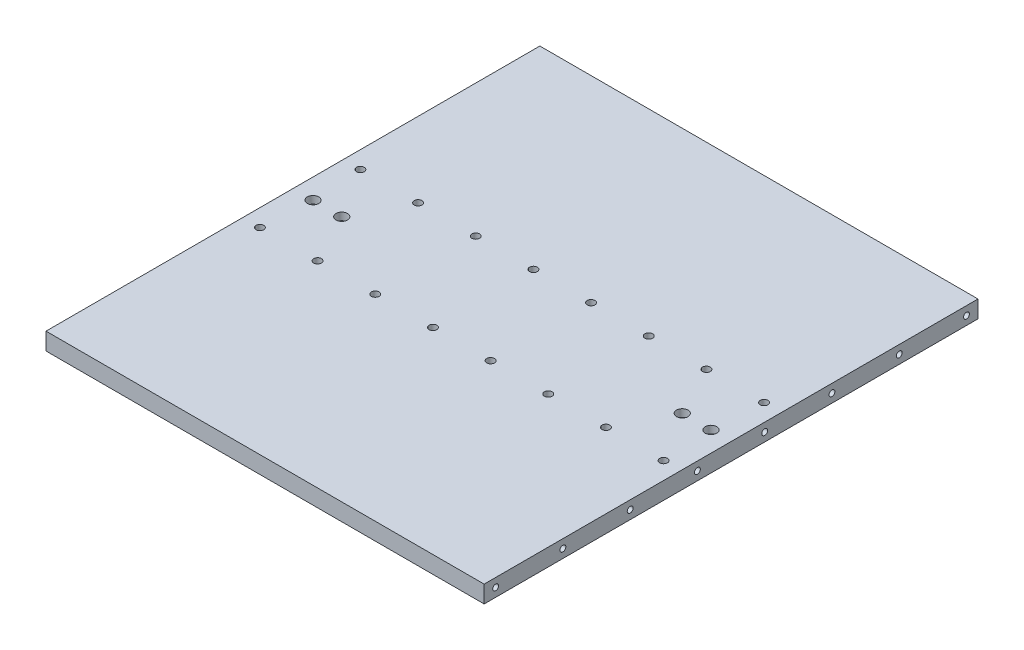
from build123d import *

# Parameters (mm, degrees)
SKETCH_1_W                = 763
SKETCH_1_H                = 860
EXTRUDE_1_DEPTH           = 30
HOLE_WIZARD_1_D           = 13.5
HOLE_WIZARD_1_CBORE_D     = 20
HOLE_WIZARD_1_CBORE_DEPTH = 13
HOLE_WIZARD_2_D           = 13.5
HOLE_WIZARD_2_CBORE_D     = 20
HOLE_WIZARD_2_CBORE_DEPTH = 13
HOLE_WIZARD_M12_1_D       = 10.2
HOLE_WIZARD_M12_1_DEPTH   = 29.25
HOLE_WIZARD_M12_1_TIP     = 3.064389157
HOLE_WIZARD_M12_2_D       = 10.2
HOLE_WIZARD_M12_2_DEPTH   = 29.25
HOLE_WIZARD_M12_2_TIP     = 3.064389157


with BuildPart() as part:
    # 草图1 → 凸台-拉伸1 (new body)
    with BuildSketch(Plane(origin=(0, 0, 0), x_dir=(1, 0, 0), z_dir=(0, 1, 0))):
        Rectangle(SKETCH_1_W, SKETCH_1_H)
    extrude(amount=EXTRUDE_1_DEPTH)

    # 打孔尺寸(%根据)内六角圆柱头螺钉的类型1 (through all)
    with Locations(Plane(origin=(0, 0, 0), x_dir=(-1, 0, 0), z_dir=(0, -1, 0))):
        with Locations((351.5, 87.5), (351.5, -87.5), (251.071428571, 87.5), (251.071428571, -87.5), (150.642857143, 87.5), (150.642857143, -87.5), (50.214285714, 87.5), (50.214285714, -87.5), (-50.214285714, -87.5), (-50.214285714, 87.5), (-150.642857143, 87.5), (-150.642857143, -87.5), (-251.071428571, 87.5), (-251.071428571, -87.5), (-351.5, -87.5), (-351.5, 87.5)):
            CounterBoreHole(HOLE_WIZARD_1_D / 2, HOLE_WIZARD_1_CBORE_D / 2, HOLE_WIZARD_1_CBORE_DEPTH)

    # 打孔尺寸(%根据)内六角圆柱头螺钉的类型2 (through all)
    with Locations(Plane(origin=(0, 30, 0), x_dir=(1, 0, 0), z_dir=(0, 1, 0))):
        with Locations((-346.5, 0), (-296.5, 0), (346.5, 0), (296.5, 0)):
            CounterBoreHole(HOLE_WIZARD_2_D / 2, HOLE_WIZARD_2_CBORE_D / 2, HOLE_WIZARD_2_CBORE_DEPTH)

    # M12 螺纹孔1
    with Locations(Plane.ZY.offset(381.5)):
        with Locations((410, 15), (292.857142857, 15), (175.714285714, 15), (58.571428571, 15), (-58.571428571, 15), (-175.714285714, 15), (-292.857142857, 15), (-410, 15)):
            Hole(HOLE_WIZARD_M12_1_D / 2, depth=HOLE_WIZARD_M12_1_DEPTH)
            with Locations((0, 0, -(HOLE_WIZARD_M12_1_DEPTH + HOLE_WIZARD_M12_1_TIP / 2))):  # 118° drill point
                Cone(0, HOLE_WIZARD_M12_1_D / 2, HOLE_WIZARD_M12_1_TIP, mode=Mode.SUBTRACT)

    # M12 螺纹孔2
    with Locations(Plane(origin=(381.5, 0, 0), x_dir=(0, 0, -1), z_dir=(1, 0, 0))):
        with Locations((-410, 15), (-292.857142857, 15), (-175.714285714, 15), (-58.571428571, 15), (58.571428571, 15), (175.714285714, 15), (292.857142857, 15), (410, 15)):
            Hole(HOLE_WIZARD_M12_2_D / 2, depth=HOLE_WIZARD_M12_2_DEPTH)
            with Locations((0, 0, -(HOLE_WIZARD_M12_2_DEPTH + HOLE_WIZARD_M12_2_TIP / 2))):  # 118° drill point
                Cone(0, HOLE_WIZARD_M12_2_D / 2, HOLE_WIZARD_M12_2_TIP, mode=Mode.SUBTRACT)


solid = part.part
